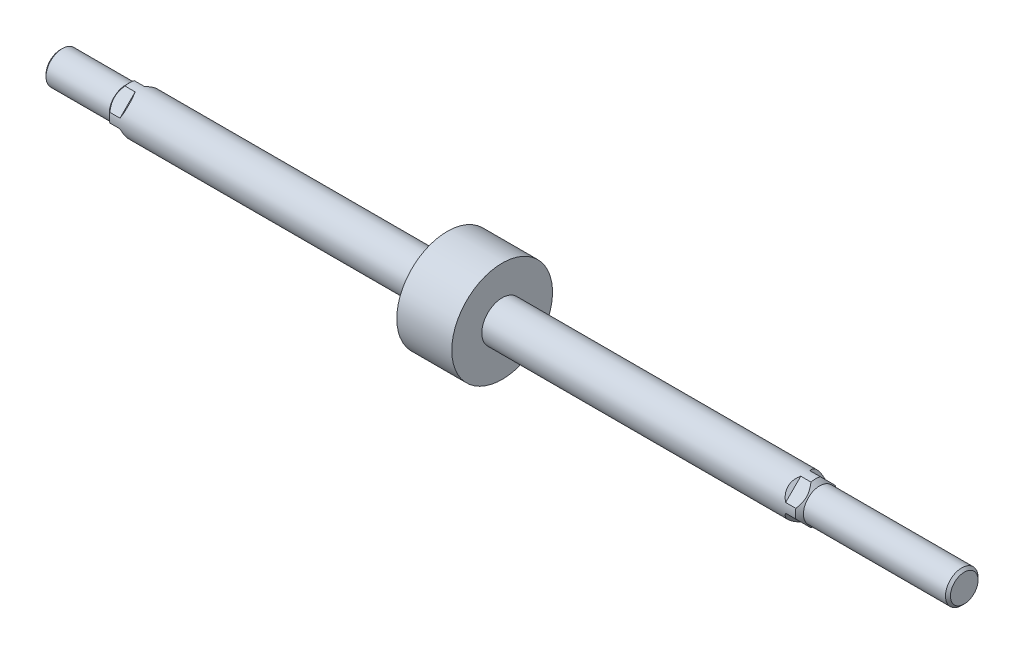
from build123d import *

# Parameters (mm, degrees)
CUT_EXTRUDE1_DEPTH      = 17
CUT_EXTRUDE1_DEPTH_BACK = 17
CUT_EXTRUDE2_DEPTH      = 17
CUT_EXTRUDE2_DEPTH_BACK = 17
CUT_EXTRUDE3_DEPTH      = 17
CUT_EXTRUDE3_DEPTH_BACK = 17
CUT_EXTRUDE4_DEPTH      = 17
CUT_EXTRUDE4_DEPTH_BACK = 17


with BuildPart() as part:
    # Sketch1 → Revolve1 (revolve)
    with BuildSketch(Plane.XY, mode=Mode.PRIVATE) as revolve1_sk:
        Polygon((-57, 0), (-57, 7.08), (-56.08, 8), (-25, 8), (-23, 10), (133, 10), (133, 24.75), (160, 24.75), (160, 0), align=None)
    revolve(revolve1_sk.sketch.rotate(Axis((160, 0, 0), (-1, 0, 0)), 270), axis=Axis((160, 0, 0), (-1, 0, 0)))

    # Sketch2 → Cut-Extrude1 (cut, two sides: drawn at the far end of the back side and taken through both)
    with BuildSketch(Plane(origin=(0, 0, 0), x_dir=(1, 0, 0), z_dir=(0, -0.7071067811865475, 0.7071067811865476)).offset(-CUT_EXTRUDE1_DEPTH_BACK)):
        Polygon((-74, -25.5), (-1, -25.5), (-18, -8.5), (-57, -8.5), (-57, 8.5), (-18, 8.5), (-1, 25.5), (-74, 25.5), align=None)
    extrude(amount=CUT_EXTRUDE1_DEPTH + CUT_EXTRUDE1_DEPTH_BACK, mode=Mode.SUBTRACT)

    # Sketch3 → Cut-Extrude2 (cut, two sides: drawn at the far end of the back side and taken through both)
    with BuildSketch(Plane(origin=(0, 0, 0), x_dir=(-1, 0, 0), z_dir=(0, -0.7071067811865476, -0.7071067811865475)).offset(-CUT_EXTRUDE2_DEPTH_BACK)):
        Polygon((74, 25.5), (1, 25.5), (18, 8.5), (57, 8.5), (57, -8.5), (18, -8.5), (1, -25.5), (74, -25.5), align=None)
    extrude(amount=CUT_EXTRUDE2_DEPTH + CUT_EXTRUDE2_DEPTH_BACK, mode=Mode.SUBTRACT)

    # Sketch4 → Revolve2 (revolve)
    with BuildSketch(Plane.XY, mode=Mode.PRIVATE) as revolve2_sk:
        Polygon((119, 0), (119, 10), (314, 10), (316, 8), (385.773, 8), (387, 6.773), (387, 0), align=None)
    revolve(revolve2_sk.sketch.rotate(Axis((387, 0, 0), (-1, 0, 0)), 270), axis=Axis((387, 0, 0), (-1, 0, 0)))

    # Sketch5 → Cut-Extrude3 (cut, two sides: drawn at the far end of the back side and taken through both)
    with BuildSketch(Plane(origin=(0, 0, 0), x_dir=(1, 0, 0), z_dir=(0, -0.7071067811865475, 0.7071067811865476)).offset(-CUT_EXTRUDE3_DEPTH_BACK)):
        Polygon((307.5, -10), (307.5, -17), (392, -17), (392, 17), (307.5, 17), (307.5, 10), (309, 8.5), (388, 8.5), (388, -8.5), (309, -8.5), align=None)
    extrude(amount=CUT_EXTRUDE3_DEPTH + CUT_EXTRUDE3_DEPTH_BACK, mode=Mode.SUBTRACT)

    # Sketch6 → Cut-Extrude4 (cut, two sides: drawn at the far end of the back side and taken through both)
    with BuildSketch(Plane(origin=(0, 0, 0), x_dir=(-1, 0, 0), z_dir=(0, -0.7071067811865476, -0.7071067811865475)).offset(-CUT_EXTRUDE4_DEPTH_BACK)):
        Polygon((-307.5, 10), (-307.5, 17), (-392, 17), (-392, -17), (-307.5, -17), (-307.5, -10), (-309, -8.5), (-388, -8.5), (-388, 8.5), (-309, 8.5), align=None)
    extrude(amount=CUT_EXTRUDE4_DEPTH + CUT_EXTRUDE4_DEPTH_BACK, mode=Mode.SUBTRACT)


solid = part.part
